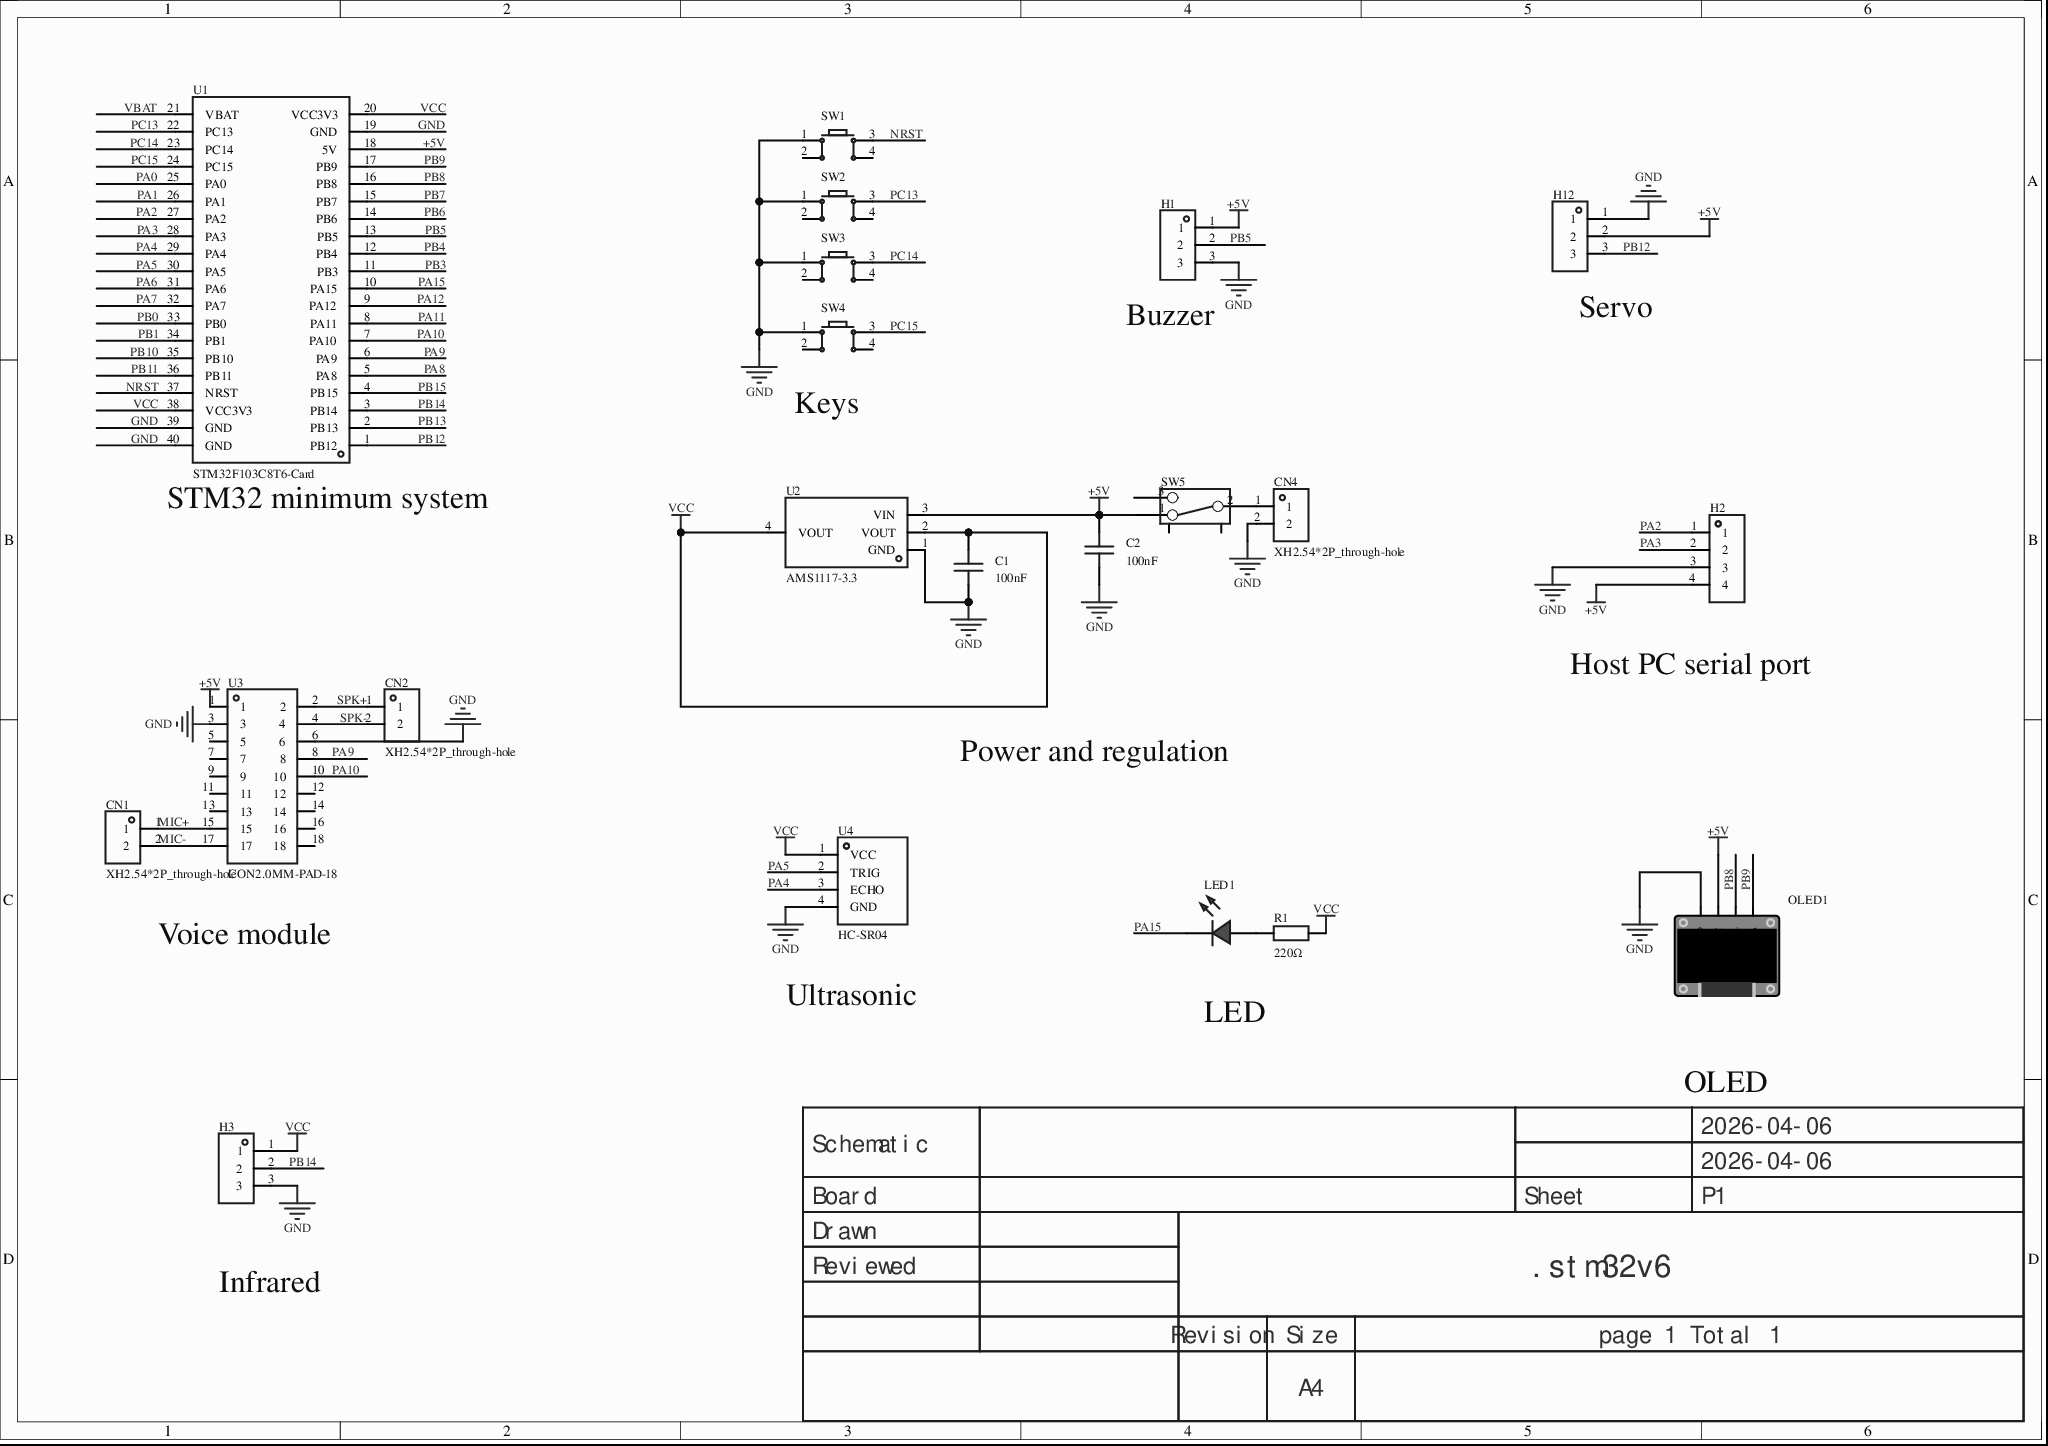
[diagram p0: MISC89011-3.schdoc]
# Altium project MISC89011-2.PrjPcb
1 sheet, 21 parts. Net scope: global (net labels, ports and power ports of the same name join across sheets).
Board file: MISC89011.pcbdoc

## Sheet MISC89011-3.schdoc
size 297 x 209 mm; Version: V1.0; @Project Name: MISC89011; @Page Count: 1; @Update Date: 2026-04-06; @Create Date: 2026-04-06; @Schematic Name: MISC89011; @Page No: 1; @Create Time: 23:22:16; @Update Time: 17:32:40; @Board Name: MISC89011

### Parts
C1  100nF  [C0603]
C2  100nF  [C0603]
CN1  XH2.54*2P_through-hole  [CONN-TH_2P-P2.50-XH2.54-2P]
CN2  XH2.54*2P_through-hole  [CONN-TH_2P-P2.50-XH2.54-2P]
CN4  XH2.54*2P_through-hole  [CONN-TH_2P-P2.50-XH2.54-2P]
H1  (no value)  [HDR-TH_3P-P2.54-V-F]
H2  (no value)  [HDR-TH_4P-P2.54-V-F]
H3  (no value)  [HDR-TH_3P-P2.54-V-F]
H12  (no value)  [HDR-TH_3P-P2.54-V-F]
LED1  (no value)  [LED_TH-3mm]
OLED1  (no value)  [0.96OLED_4P]
R1  220Ω  [Res_1/8W]
SW1  (no value)  [SW-TH_4P-L6.0-W6.0-P4.50-LS6.5]
SW2  (no value)  [SW-TH_4P-L6.0-W6.0-P4.50-LS6.5]
SW3  (no value)  [SW-TH_4P-L6.0-W6.0-P4.50-LS6.5]
SW4  (no value)  [SW-TH_4P-L6.0-W6.0-P4.50-LS6.5]
SW5  (no value)  [拨动开关]
U1  STM32F103C8T6-Card  [CONN-TH_L53.3-W22.9_STM32F103C8T6-CARD]
U2  AMS1117-3.3  [SOT-223-3_L6.5-W3.4-P2.30-LS7.0-BR]
U3  CON2.0MM-PAD-18  [CONN-TH_18P-P2.00_C9900078766]
U4  HC-SR04  [TH_HC-SR04V]

### Nets
+5V: C2.2 H1.1 H2.4 H12.2 OLED1.2(VCC) SW5.1 U1.18(5V) U2.3(VIN) U3.1
GND: C1.1 C2.1 CN4.2 H1.3 H2.3 H3.3 H12.1 OLED1.1(GND) SW1.1 SW2.1 SW3.1 SW4.1 U1.19(GND) U1.39(GND) U1.40(GND) U2.1(GND) U3.3 U3.6 U4.4(GND)
VCC: C1.2 H3.1 R1.2 U1.20(VCC3V3) U1.38(VCC3V3) U2.2(VOUT) U2.4(VOUT) U4.1(VCC)
MIC+: CN1.1 U3.15
MIC-: CN1.2 U3.17
NRST: SW1.3 U1.37(NRST)
PA0: U1.25(PA0)
PA1: U1.26(PA1)
PA2: H2.1 U1.27(PA2)
PA3: H2.2 U1.28(PA3)
PA4: U1.29(PA4) U4.3(ECHO)
PA5: U1.30(PA5) U4.2(TRIG)
PA6: U1.31(PA6)
PA7: U1.32(PA7)
PA8: U1.5(PA8)
PA9: U1.6(PA9) U3.8
PA10: U1.7(PA10) U3.10
PA11: U1.8(PA11)
PA12: U1.9(PA12)
PA15: LED1.2(A) U1.10(PA15)
PB0: U1.33(PB0)
PB1: U1.34(PB1)
PB3: U1.11(PB3)
PB4: U1.12(PB4)
PB5: H1.2 U1.13(PB5)
PB6: U1.14(PB6)
PB7: U1.15(PB7)
PB8: OLED1.3(SCL) U1.16(PB8)
PB9: OLED1.4(SDA) U1.17(PB9)
PB10: U1.35(PB10)
PB11: U1.36(PB11)
PB12: H12.3 U1.1(PB12)
PB13: U1.2(PB13)
PB14: H3.2 U1.3(PB14)
PB15: U1.4(PB15)
PC13: SW2.3 U1.22(PC13)
PC14: SW3.3 U1.23(PC14)
PC15: SW4.3 U1.24(PC15)
SPK+: CN2.1 U3.2
SPK-: CN2.2 U3.4
VBAT: U1.21(VBAT)
NetCN4_1: CN4.1 SW5.2
NetLED1_1: LED1.1(C) R1.1

Not connected (* = marked no-connect by the designer): SW1 2 4; SW2 2 4; SW3 2 4; SW4 2 4; SW5 3 4 5; U3 5 7 9 11 12 13 14 16 18

### Notes on the sheet
- (near H1) Buzzer
- (near H12) Servo
- (near SW4) Keys
- (near U1) STM32 minimum system
- (near H2) Host PC serial port
- Power and regulation
- Voice module
- Ultrasonic
- LED
- OLED
- Infrared
- 2026-04-06
- Schematic
- Board
- Sheet
- P1
- Drawn
- Reviewed
- .stm32v6
- Revision
- Size
- A4
- page 1 Total 1

### Library data of the parts
C1 C2 = CAP_0603: Symbol: Capacitance; ConvertToPcb: yes; ModelId: ac125912035d415993ca9572d50418b10819f05c4eef4c71ace90d822a990e87; ModelName: C0603_L1.6-W0.8-H0.8; ModelTransform: 62.992,31.496,0,0,0,0,0,0,0; Device: CAP_0603; AddInBom: yes; Supplier Footprint: 0603; FootprintName: C0603; Value: 100nF
CN1 CN2 CN4 = XH2.54*2P_直插: 3D Model: 325c595e30db4df8abe76612dd40b0fa0819f05c4eef4c71ace90d822a990e87; 3D Model Transform: 295.275,228.346,0,180,0,0,-0.002,-20.079,-137.795; AddInBom: yes; Symbol: XH2.54*2P_through-hole; Device: XH2.54*2P_through-hole; LCSC Part Name: XH2.54*2P_直插; Supplier Part: C9900008615; Manufacturer Part: XH2.54*2P_直插; Supplier Footprint: XH2.54_2P; JLCPCB Part Class: Extended Part; Supplier: LCSC; ConvertToPcb: yes; FootprintName: CONN-TH_2P-P2.50-XH2.54-2P; ModelName: CONN-TH_2P-P2.50-XH2.54-2P
H1 H3 H12 = HDR-F_2.54_1x3P: Symbol: PM254V-11-03-H85; 3D Model: f3b3cc5aae9641bf9e56fc160cef875b; 3D Model Transform: 299.9994,100,0,0,0,0,0,0,-118.11; ConvertToPcb: yes; ModelName: HDR2.54-F-LI-1X3P; Device: HDR-F_2.54_1x3P; Supplier Part: C541850; Supplier Footprint: 插件; AddInBom: yes; FootprintName: HDR-TH_3P-P2.54-V-F
H2 = HDR-F_2.54_1x4P: Symbol: 2.54-1*4P female; ConvertToPcb: yes; ModelId: d187812051054f85879fcaa51a310d8e0819f05c4eef4c71ace90d822a990e87; ModelTransform: 419.6842,98.464,0,0,0,0,0,0,-118.11; Device: HDR-F_2.54_1x4P; AddInBom: yes; SupplierPart: C2718488; Supplier Footprint: 插件; FootprintName: HDR-TH_4P-P2.54-V-F; ModelName: HDR-TH_4P-P2.54-V-F
LED1 = LED_TH-R_3mm: 3D Model: a497c992633541038a38947cdc58012f0819f05c4eef4c71ace90d822a990e87; 3D Model Transform: 141.274,153.327,0,0,0,0,-5.984,0,-137.795; ConvertToPcb: yes; ModelName: LED-TH-3mm_R; Symbol: LED_TH-R; Device: LED_TH-R_3mm; Supplier Footprint: 插件; AddInBom: yes; FootprintName: LED_TH-3mm
OLED1 = 0.96OLED模块_4P: Symbol: 0.96OLED module_4P; ConvertToPcb: yes; ModelId: 79c000fdb68d45a296c2e9bedf4f9055; ModelTransform: 1393.69792,1318.895,0,0,0,0,0,-560.079,-137.795; Device: 0.96OLED module_4P; AddInBom: yes; FootprintName: 0.96OLED_4P; Supplier Footprint: 插件; ModelName: 0.96OLED_4P
R1 = Res_AXIAL-1/8W: Symbol: Resistor; 3D Model: b2b5ae7ae4c642178fe0039925c86a3f0819f05c4eef4c71ace90d822a990e87; 3D Model Transform: 282.86,66.88,253.09,0,0,0,0,0,-191; ConvertToPcb: yes; ModelName: RES-TH_BD1.8-L3.2-P7.20-D0.4; Device: Res_AXIAL-1/8W; Value: 220Ω; Supplier Footprint: 轴向引线; AddInBom: yes; FootprintName: Res_1/8W
SW1-SW4 = Key_TH_6x6x6: Contact current: 50mA; rated voltage (DC): 12V; insulation resistance: 100MΩ; circuit: SPST; mounting: through-hole; button shape: round; button/cap colour: black; actuating force: 260gf@±30gf; operating temperature: -25℃~+70℃; pin style: PC pin; switch length: 6mm; switch width: 6mm; switch height: 6mm; with bracket: no;; Symbol: Tactile switch; AddInBom: yes; ModelId: 20eee248bc684ccd8cbdbb1d0d91ec6f0819f05c4eef4c71ace90d822a990e87; ModelName: SW-TH_4P-L6.0-W6.0-H5.0-LS6.5-P4.50; ModelTransform: 236.22,323.03,0,90,0,0,0,0,-137.795; Device: Key_TH_6x6x6; ConvertToPcb: yes; FootprintName: SW-TH_4P-L6.0-W6.0-P4.50-LS6.5; Supplier Footprint: 插件
SW5 = 拨动开关_正: Symbol: Toggle switch; Device: Toggle switch_pos; ConvertToPcb: yes; ModelId: 4321fe59a4074cbfb4989553f297c68f0819f05c4eef4c71ace90d822a990e87; ModelName: SW-TH_SS-12D02-VG4; ModelTransform: 370.09,208.7,472.35,0,0,0,0,0,-110; AddInBom: yes; Supplier Footprint: 插件; FootprintName: Toggle switch
U1 = STM32F103C8T6-Card: AddInBom: yes; Symbol: STM32F103C8T6-CARD; Device: STM32F103C8T6-Card; LCSC Part Name: STM32F103C8T6-Card; SupplierPart: C9900077949; ManufacturerPart: STM32F103C8T6-Card; Supplier Footprint: 插件; Supplier: LCSC; ConvertToPcb: yes; FootprintName: CONN-TH_L53.3-W22.9_STM32F103C8T6-CARD
U2 = AMS1117-3.3_C6186: Output type: fixed; working voltage: -; output voltage: 3.3V; output current: 1A; PSRR: 72dB@(120Hz); output polarity: positive;; Manufacturer: AMS; AddInBom: yes; ModelId: 925194bf9823436183a3e0b978a8d076; ModelName: SOT-223-4P_L6.5-W3.5-H1.6-LS7.0-P2.30; ModelTransform: 279.89794,255.905,0,180,0,0,-3.9385,-0.0005,0; Voltage Dropout: 1.3V@(800mA); Number of Outputs: 1; Symbol: AMS1117-3.3; Device: AMS1117-3.3_C6186; LCSC Part Name: 输出3.3V 1A; SupplierPart: C6186; ManufacturerPart: AMS1117-3.3; Supplier Footprint: SOT-223; Datasheet: https://atta.szlcsc.com/upload/public/pdf/source/20180727/C6186_7A095716F0823C02F1997A905E26C086.pdf; Supplier: LCSC; ConvertToPcb: yes; FootprintName: SOT-223-3_L6.5-W3.4-P2.30-LS7.0-BR; Output Type: Fixed; Voltage - Supply: -; Output Voltage: 3.3V; Output Current: 1A; Power Supply Rejection Ratio (PSRR): 72dB@(120Hz); standby current: -; Noise: -; Features: Overcurrent protection (OCP); thermal shutdown (TSD); Operating Temperature: -; Output Configuration: Positive
U3 = CON2.0MM-PAD-18: 3D Model: 07100c6dd3a4442ea12d6f5a4e41c4c80819f05c4eef4c71ace90d822a990e87; 3D Model Transform: 787.7937,374.015,0,0,0,0,0,-14.961,-118.11; AddInBom: yes; Symbol: CON2.0MM-PAD-18; Device: CON2.0MM-PAD-18; LCSC Part Name: CON2.0MM-PAD-18; Supplier Part: C9900078766; Manufacturer Part: CON2.0MM-PAD-18; Supplier Footprint: TH-2*9P-2.0; JLCPCB Part Class: Extended Part; Supplier: LCSC; ConvertToPcb: yes; FootprintName: CONN-TH_18P-P2.00_C9900078766; ModelName: CONN-TH_18P-P2.00_C9900078766
U4 = HC-SR04: Manufacturer: Universal Microelectronics; AddInBom: yes; Symbol: HC-SR04; Device: HC-SR04; LCSC Part Name: HC-SR04; Supplier Part: C19857336; Manufacturer Part: HC-SR04; Supplier Footprint: -; JLCPCB Part Class: Extended library; Datasheet: https://atta.szlcsc.com/upload/public/pdf/source/20240122/47B8E374E428935B7962A2189EF91AAC.pdf; Supplier: LCSC; ConvertToPcb: yes; FootprintName: TH_HC-SR04V